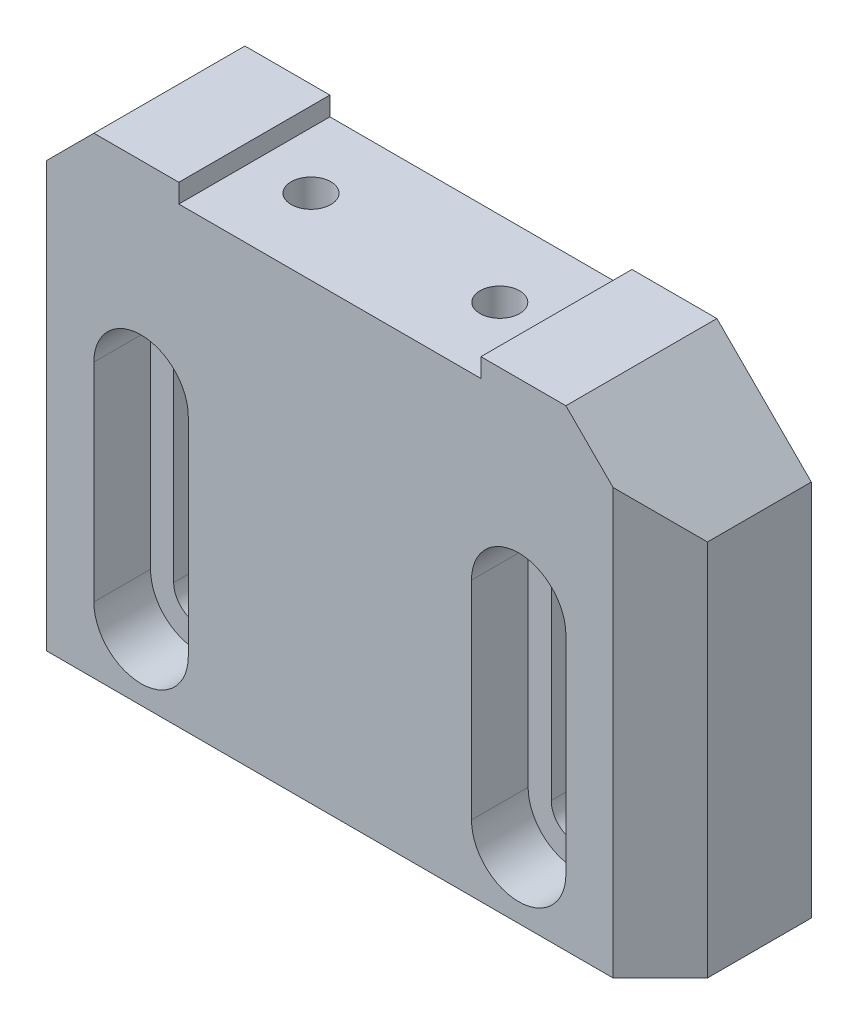
SolidWorks part; units mm, degrees
material "A6061"
ref_plane "前视基准面" through (0, 0, 0) normal (0, 0, 1) x (1, 0, 0)
ref_plane "上视基准面" through (0, 0, 0) normal (0, 1, 0) x (1, 0, 0)
ref_plane "右视基准面" through (0, 0, 0) normal (1, 0, 0) x (0, 0, -1)
sketch "Sketch1" plane through (0, 0, 0) normal (0, 0, 1) x (1, 0, 0)
  line L1 (35, -25) -> (-35, -25)
  line L2 (35, -25) -> (35, 25)
  line L3 (35, 25) -> (-35, 25)
  line L4 (-35, -25) -> (-35, 25)
  line L5 (35, -25) -> (-35, 25) construction
  line L6 (35, 25) -> (-35, -25) construction
  point P0 (0, 0)
  dimension "D1" = 70
  dimension "D2" = 50
extrude "Extrude1" add sketch "Sketch1" along normal mid plane 16
sketch "Sketch2" plane through (0, 25, 0) normal (0, 1, 0) x (1, 0, 0)
  line L0 (35, 8) -> (-35, 8) construction
  line L1 (16, -8) -> (-16, -8)
  line L2 (16, -8) -> (16, 8)
  line L3 (16, 8) -> (-16, 8)
  line L4 (-16, -8) -> (-16, 8)
  line L5 (16, -8) -> (-16, 8) construction
  line L6 (16, 8) -> (-16, -8) construction
  point P0 (0, 0)
  dimension "D1" = 32
extrude "Extrude2" cut sketch "Sketch2" against normal blind 2
hole_wizard "M5 Tapped Hole1" positions "Sketch4" profile "Sketch3" tap size "M5" standard "ISO"
sketch "Sketch4" plane through (0, 23, 0) normal (0, 1, 0) x (1, 0, 0)
  line L0 (-10, 0) -> (10, 0) construction
  point P0 (-10, 0)
  point P2 (10, 0)
  dimension "D1" = 20
sketch "Sketch3" plane through (-10, 23, 0) normal (1, 0, 0) x (0, 0, 1)
  line L0 (0, 0) -> (0, 9.6618)
  line L1 (0, 9.6618) -> (2.1, 8.4)
  line L2 (2.1, 8.4) -> (2.1, 0)
  line L5 (2.1, 0) -> (0, 0)
  line L10 (0, 9.6618) -> (-2.1, 8.4) construction
  line L11 (0, -6.35) -> (0, 107.95) construction
  dimension "螺纹孔钻头直径" = 4.2
  dimension "螺纹孔钻头深度" = 8.4
  dimension "导头角度" = 118
cosmetic thread "Cosmetic Thread1" parameters "D1"=6, "D2"=5
cosmetic thread "Cosmetic Thread2" parameters "D1"=6, "D2"=5
sketch "Sketch5" plane through (0, 0, -8) normal (0, 0, 1) x (1, 0, 0)
  line L0 (-35, -25) -> (35, -25) construction
  line L1 (-33, -25) -> (33, -25)
  line L2 (-33, -25) -> (-33, 7)
  line L3 (-30, 10) -> (30, 10)
  line L4 (33, -25) -> (33, 7)
  line L5 (0, 0) -> (0, 10) construction
  arc A0 (30, 10) -> (33, 7) centre (30, 7) cw
  arc A1 (-33, 7) -> (-30, 10) centre (-30, 7) cw
  point P13 (-33, 10)
  dimension "D3" = 3
  dimension "D1" = 66
  dimension "D2" = 35
extrude "Extrude3" cut sketch "Sketch5" along normal blind 8
sketch "Sketch6" plane through (0, 0, 8) normal (0, 0, 1) x (1, 0, 0)
  line L0 (-20, -18) -> (-20, 4) construction
  line L1 (-22.55, -18) -> (-22.55, 4)
  line L2 (-17.45, -18) -> (-17.45, 4)
  line L3 (20, -18) -> (20, 4) construction
  line L4 (17.45, -18) -> (17.45, 4)
  line L5 (22.55, -18) -> (22.55, 4)
  line L6 (-20, -7) -> (20, -7) construction
  line L7 (0, -25) -> (0, -7) construction
  line L8 (-35, -25) -> (35, -25) construction
  arc A0 (-22.55, -18) -> (-17.45, -18) centre (-20, -18) ccw
  arc A1 (-17.45, 4) -> (-22.55, 4) centre (-20, 4) ccw
  arc A2 (17.45, -18) -> (22.55, -18) centre (20, -18) ccw
  arc A3 (22.55, 4) -> (17.45, 4) centre (20, 4) ccw
  point P2 (-20, -7)
  point P7 (20, -7)
  dimension "D2" = 2.55
  dimension "D1" = 40
  dimension "D3" = 22
  dimension "D4" = 18
extrude "Extrude4" cut sketch "Sketch6" against normal through all
sketch "Sketch7" plane through (0, 0, 8) normal (0, 0, 1) x (1, 0, 0)
  line L0 (20, -18) -> (20, 4) construction
  line L1 (15, -18) -> (15, 4)
  line L2 (25, -18) -> (25, 4)
  line L3 (-20, 4) -> (-20, -18) construction
  line L4 (-15, 4) -> (-15, -18)
  line L5 (-25, 4) -> (-25, -18)
  arc A0 (15, -18) -> (25, -18) centre (20, -18) ccw
  arc A1 (25, 4) -> (15, 4) centre (20, 4) ccw
  arc A2 (-15, 4) -> (-25, 4) centre (-20, 4) ccw
  arc A3 (-25, -18) -> (-15, -18) centre (-20, -18) ccw
  point P4 (20, -7)
  point P9 (-20, -7)
  dimension "D1" = 5
extrude "Extrude5" cut sketch "Sketch7" against normal blind 6
chamfer "Chamfer1" distance 10 angle 45 2 edges at (-35, 25, 0) (35, 25, 0)
chamfer "Chamfer2" distance 5 angle 45 2 edges at (-35, -5, 8) (35, -5, 8)
